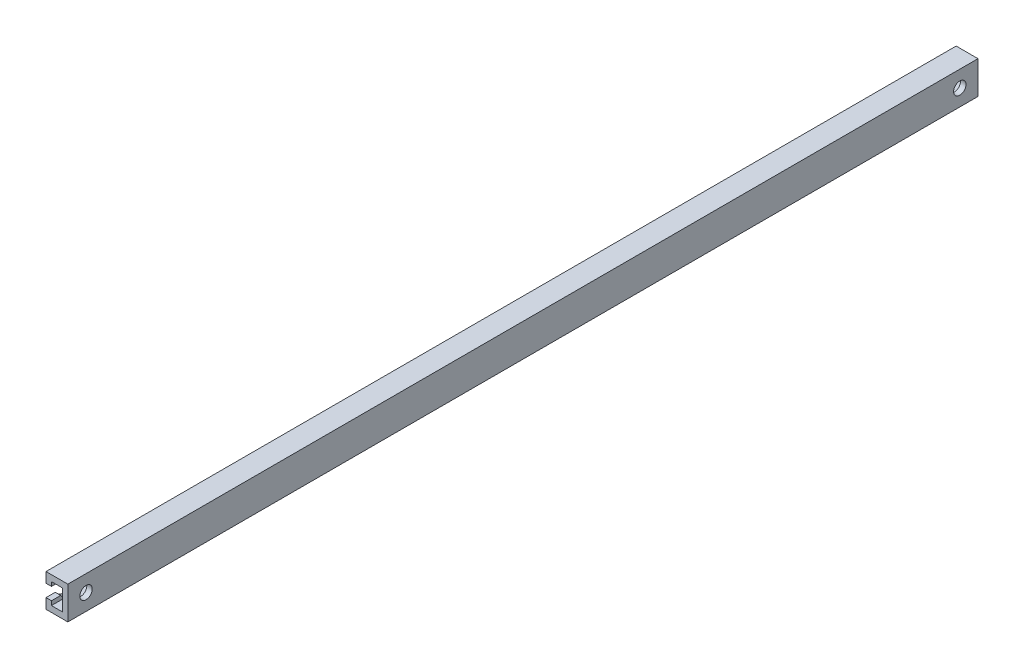
from build123d import *

# Parameters (mm, degrees)
EXTRUDE_1_DEPTH           = 250
HOLE_WIZARD_1_D           = 3.4
HOLE_WIZARD_1_CBORE_D     = 6
HOLE_WIZARD_1_CBORE_DEPTH = 3.4


with BuildPart() as part:
    # 草圖1 → 伸長1 (new body)
    with BuildSketch(Plane.XY):
        Polygon((-3, 4.5), (3, 4.5), (3, -4.5), (-3, -4.5), (-3, -1.7), (-1.5, -1.7), (-1.5, -2.85), (1.5, -2.85), (1.5, 2.85), (-1.5, 2.85), (-1.5, 1.7), (-3, 1.7), align=None)
    extrude(amount=EXTRUDE_1_DEPTH)

    # 打孔尺寸(%根据)内六角圆柱头螺钉的类型1 (through all)
    with Locations(Plane.ZY.offset(3)):
        with Locations((245, 0), (5, 0)):
            CounterBoreHole(HOLE_WIZARD_1_D / 2, HOLE_WIZARD_1_CBORE_D / 2, HOLE_WIZARD_1_CBORE_DEPTH)


solid = part.part
